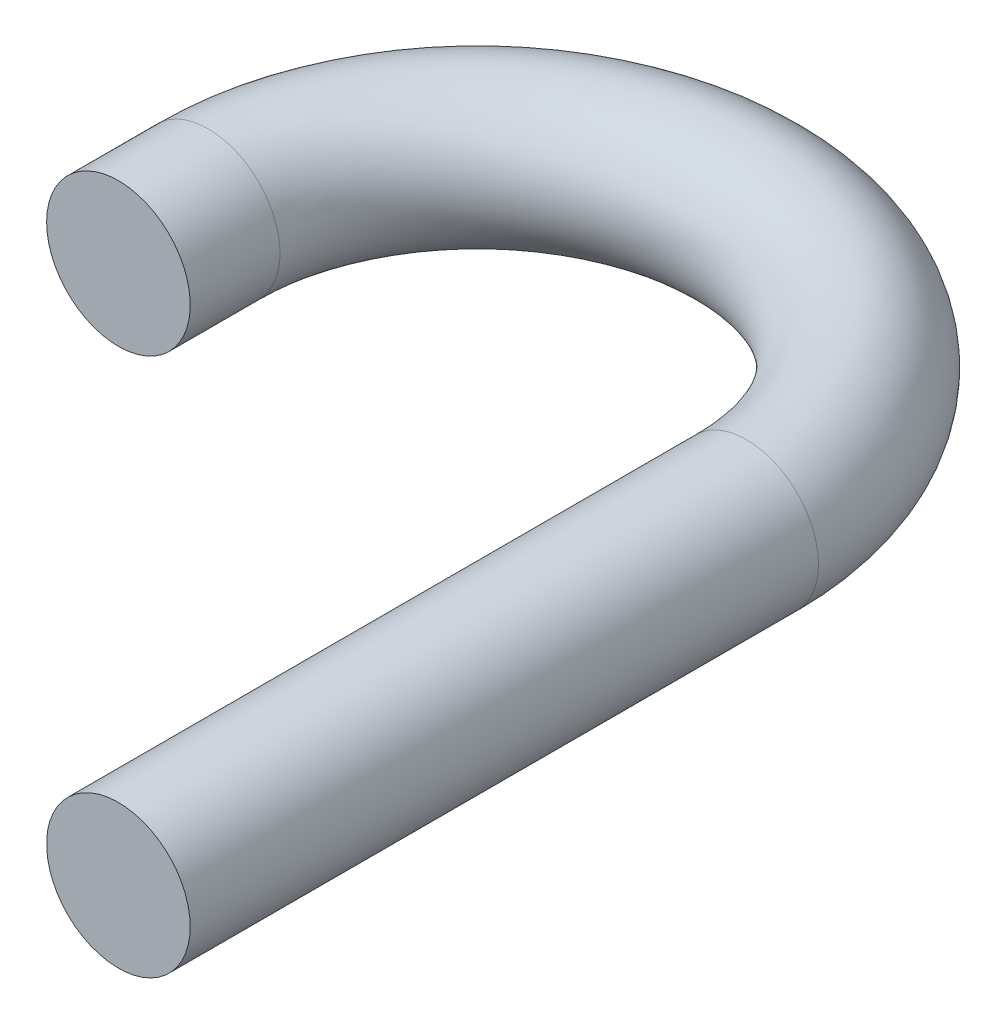
from build123d import *

# Parameters (mm, degrees)
SKETCH1_R = 8


with BuildPart() as part:
    # Sweep1: sweep along a path in Sketch2
    with BuildLine(Plane(origin=(0, 0, 0), x_dir=(1, 0, 0), z_dir=(0, 1, 0))) as sweep1_path:
        Line((0, 0), (0, 70))
        ThreePointArc((0, 70), (-30, 100), (-60, 70))
        Line((-60, 70), (-60, 60))
    # Sketch1 → Sweep1 (sweep)
    with BuildSketch(Plane.XY):
        Circle(SKETCH1_R)
    sweep(path=sweep1_path.line)


solid = part.part
